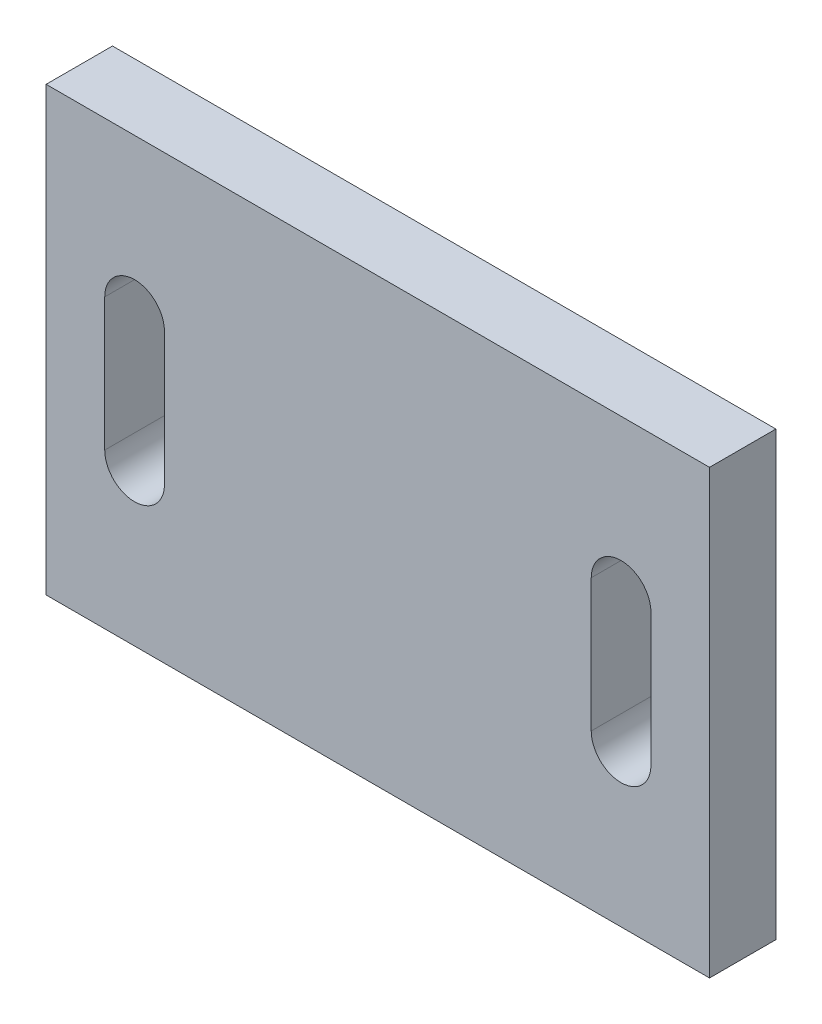
from build123d import *

# Parameters (mm, degrees)
SKETCH1_W           = 300
SKETCH1_H           = 200
BOSS_EXTRUDE1_DEPTH = 30


with BuildPart() as part:
    # Sketch1 → Boss-Extrude1 (new body)
    with BuildSketch(Plane.XY):
        with Locations((150, 100)):
            Rectangle(SKETCH1_W, SKETCH1_H)
        with BuildLine():
            Line((273.5, 130), (273.5, 70))
            ThreePointArc((273.5, 70), (260, 56.5), (246.5, 70))
            Line((246.5, 70), (246.5, 130))
            ThreePointArc((246.5, 130), (260, 143.5), (273.5, 130))
        make_face(mode=Mode.SUBTRACT)
        with BuildLine():
            Line((53.5, 130), (53.5, 70))
            ThreePointArc((53.5, 70), (40, 56.5), (26.5, 70))
            Line((26.5, 70), (26.5, 130))
            ThreePointArc((26.5, 130), (40, 143.5), (53.5, 130))
        make_face(mode=Mode.SUBTRACT)
    extrude(amount=BOSS_EXTRUDE1_DEPTH)


solid = part.part
